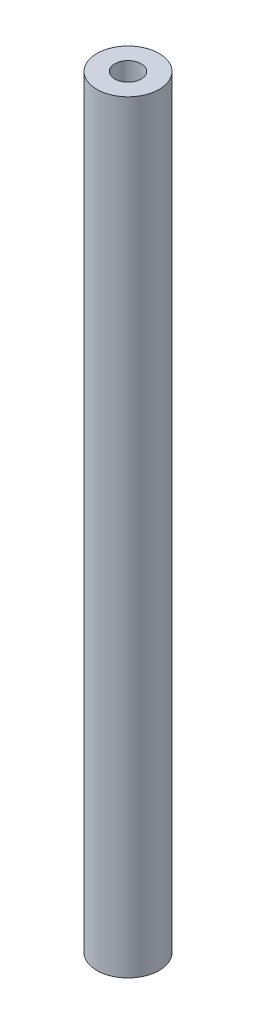
from build123d import *

# Parameters (mm, degrees)
SKETCH_1_W             = 8
SKETCH_1_H             = 196
HOLE_WIZARD_M8_1_D     = 6.8
HOLE_WIZARD_M8_1_DEPTH = 8
HOLE_WIZARD_M8_1_TIP   = 2.042926105
HOLE_WIZARD_M8_2_D     = 6.8
HOLE_WIZARD_M8_2_DEPTH = 8
HOLE_WIZARD_M8_2_TIP   = 2.042926105


with BuildPart() as part:
    # 草图1 → 旋转-薄壁1 (revolve)
    with BuildSketch(Plane.XY, mode=Mode.PRIVATE) as revolve_1_sk:
        with Locations((-4, 98)):
            Rectangle(SKETCH_1_W, SKETCH_1_H)
    revolve(revolve_1_sk.sketch.rotate(Axis((0, 0, 0), (0, 1, 0)), 270), axis=Axis((0, 0, 0), (0, 1, 0)))

    # M8 螺纹孔的螺纹孔钻头1
    with Locations(Plane(origin=(0, 0, 0), x_dir=(-1, 0, 0), z_dir=(0, -1, 0))):
        with Locations((0, 0)):
            Hole(HOLE_WIZARD_M8_1_D / 2, depth=HOLE_WIZARD_M8_1_DEPTH)
            with Locations((0, 0, -(HOLE_WIZARD_M8_1_DEPTH + HOLE_WIZARD_M8_1_TIP / 2))):  # 118° drill point
                Cone(0, HOLE_WIZARD_M8_1_D / 2, HOLE_WIZARD_M8_1_TIP, mode=Mode.SUBTRACT)

    # M8 螺纹孔的螺纹孔钻头2
    with Locations(Plane(origin=(0, 196, 0), x_dir=(1, 0, 0), z_dir=(0, 1, 0))):
        with Locations((0, 0)):
            Hole(HOLE_WIZARD_M8_2_D / 2, depth=HOLE_WIZARD_M8_2_DEPTH)
            with Locations((0, 0, -(HOLE_WIZARD_M8_2_DEPTH + HOLE_WIZARD_M8_2_TIP / 2))):  # 118° drill point
                Cone(0, HOLE_WIZARD_M8_2_D / 2, HOLE_WIZARD_M8_2_TIP, mode=Mode.SUBTRACT)


solid = part.part
